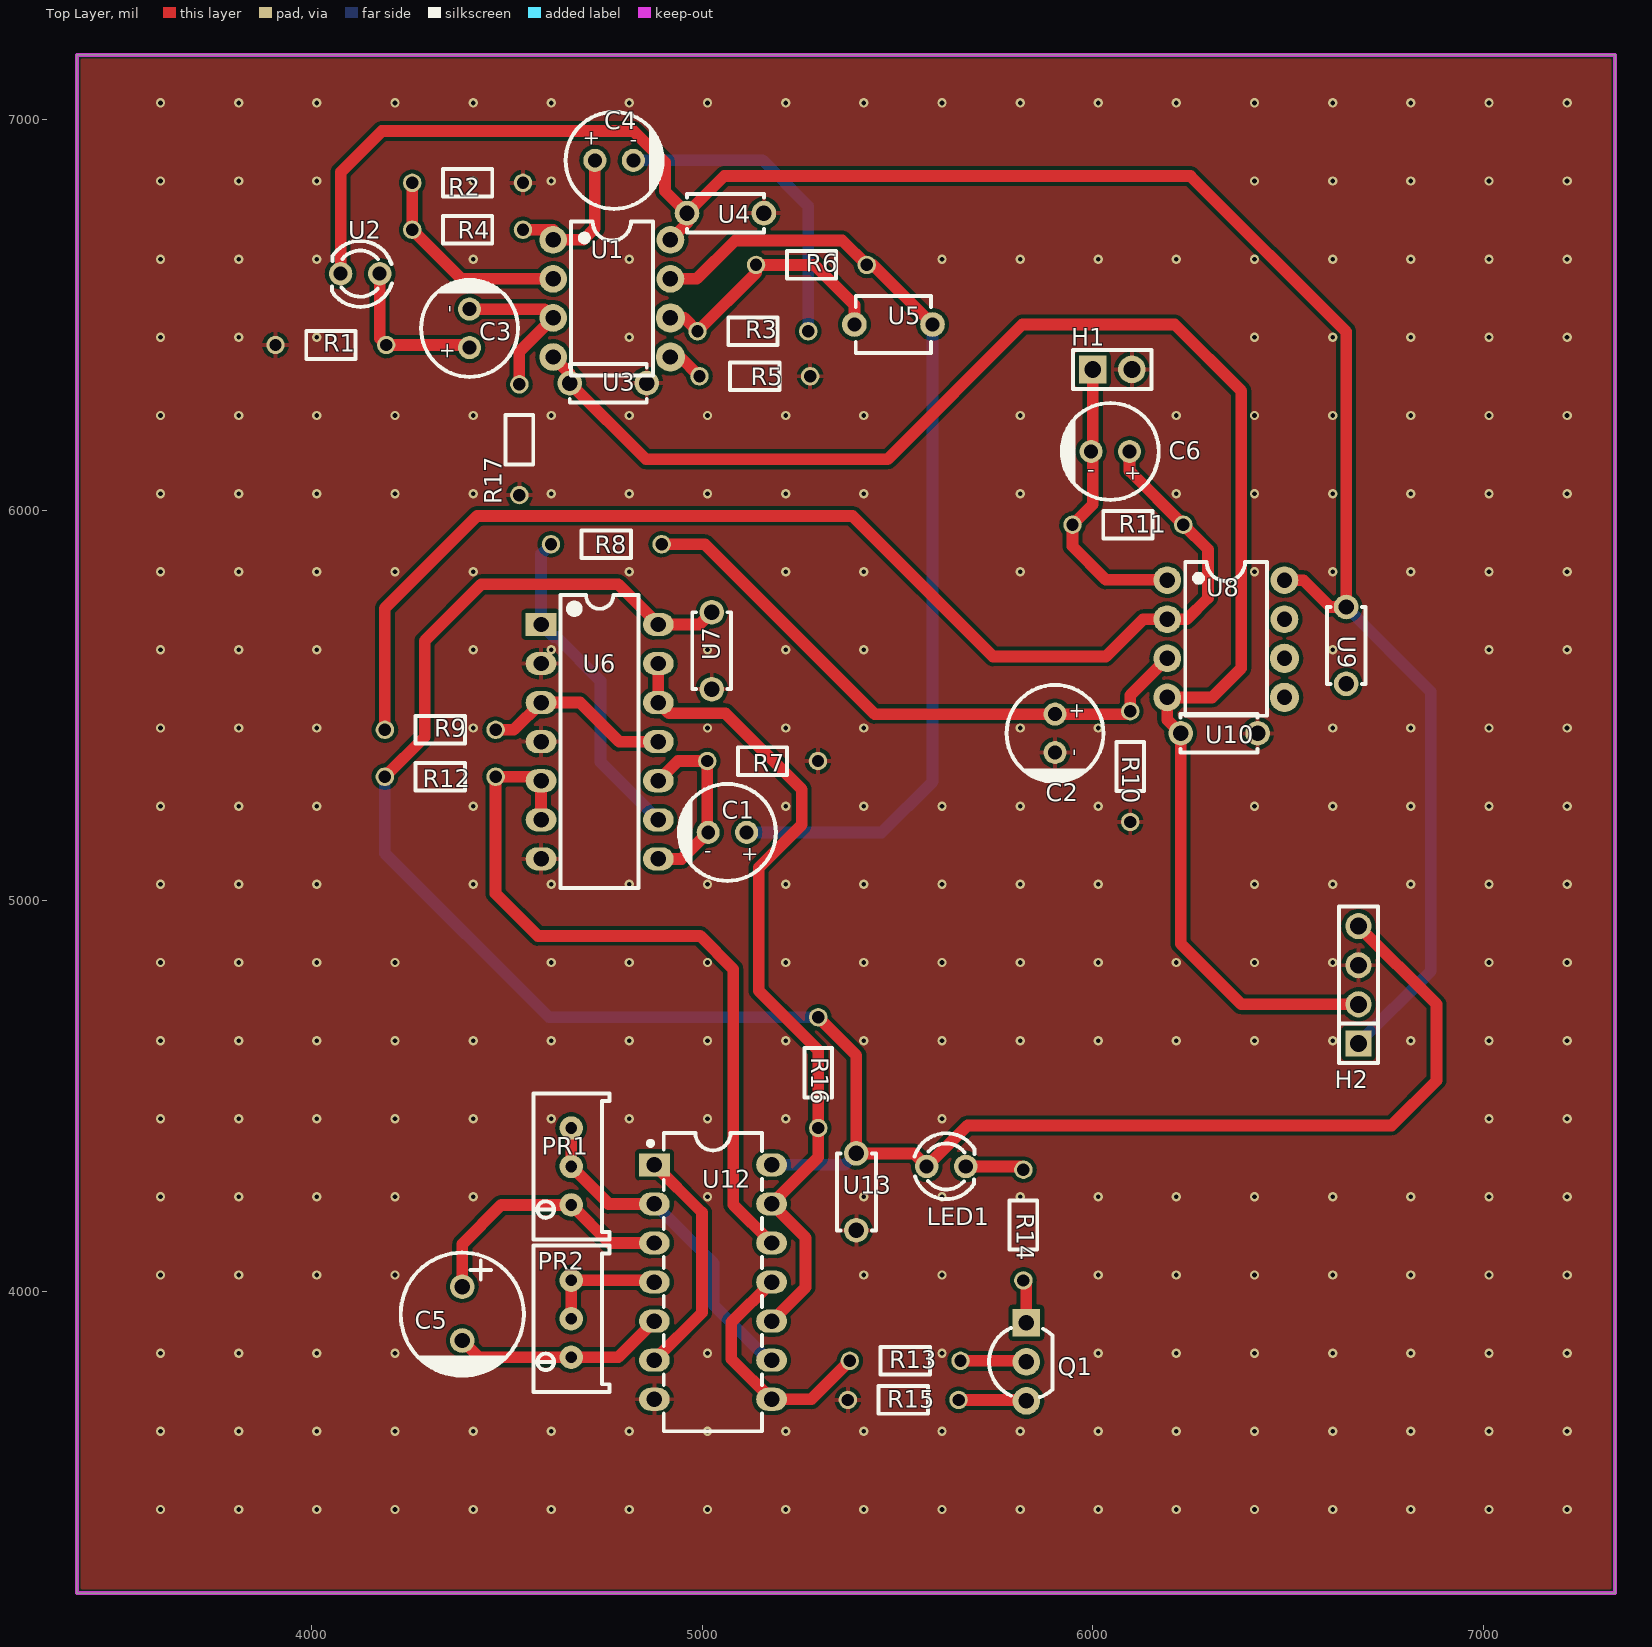
[diagram p0: Top Layer view]
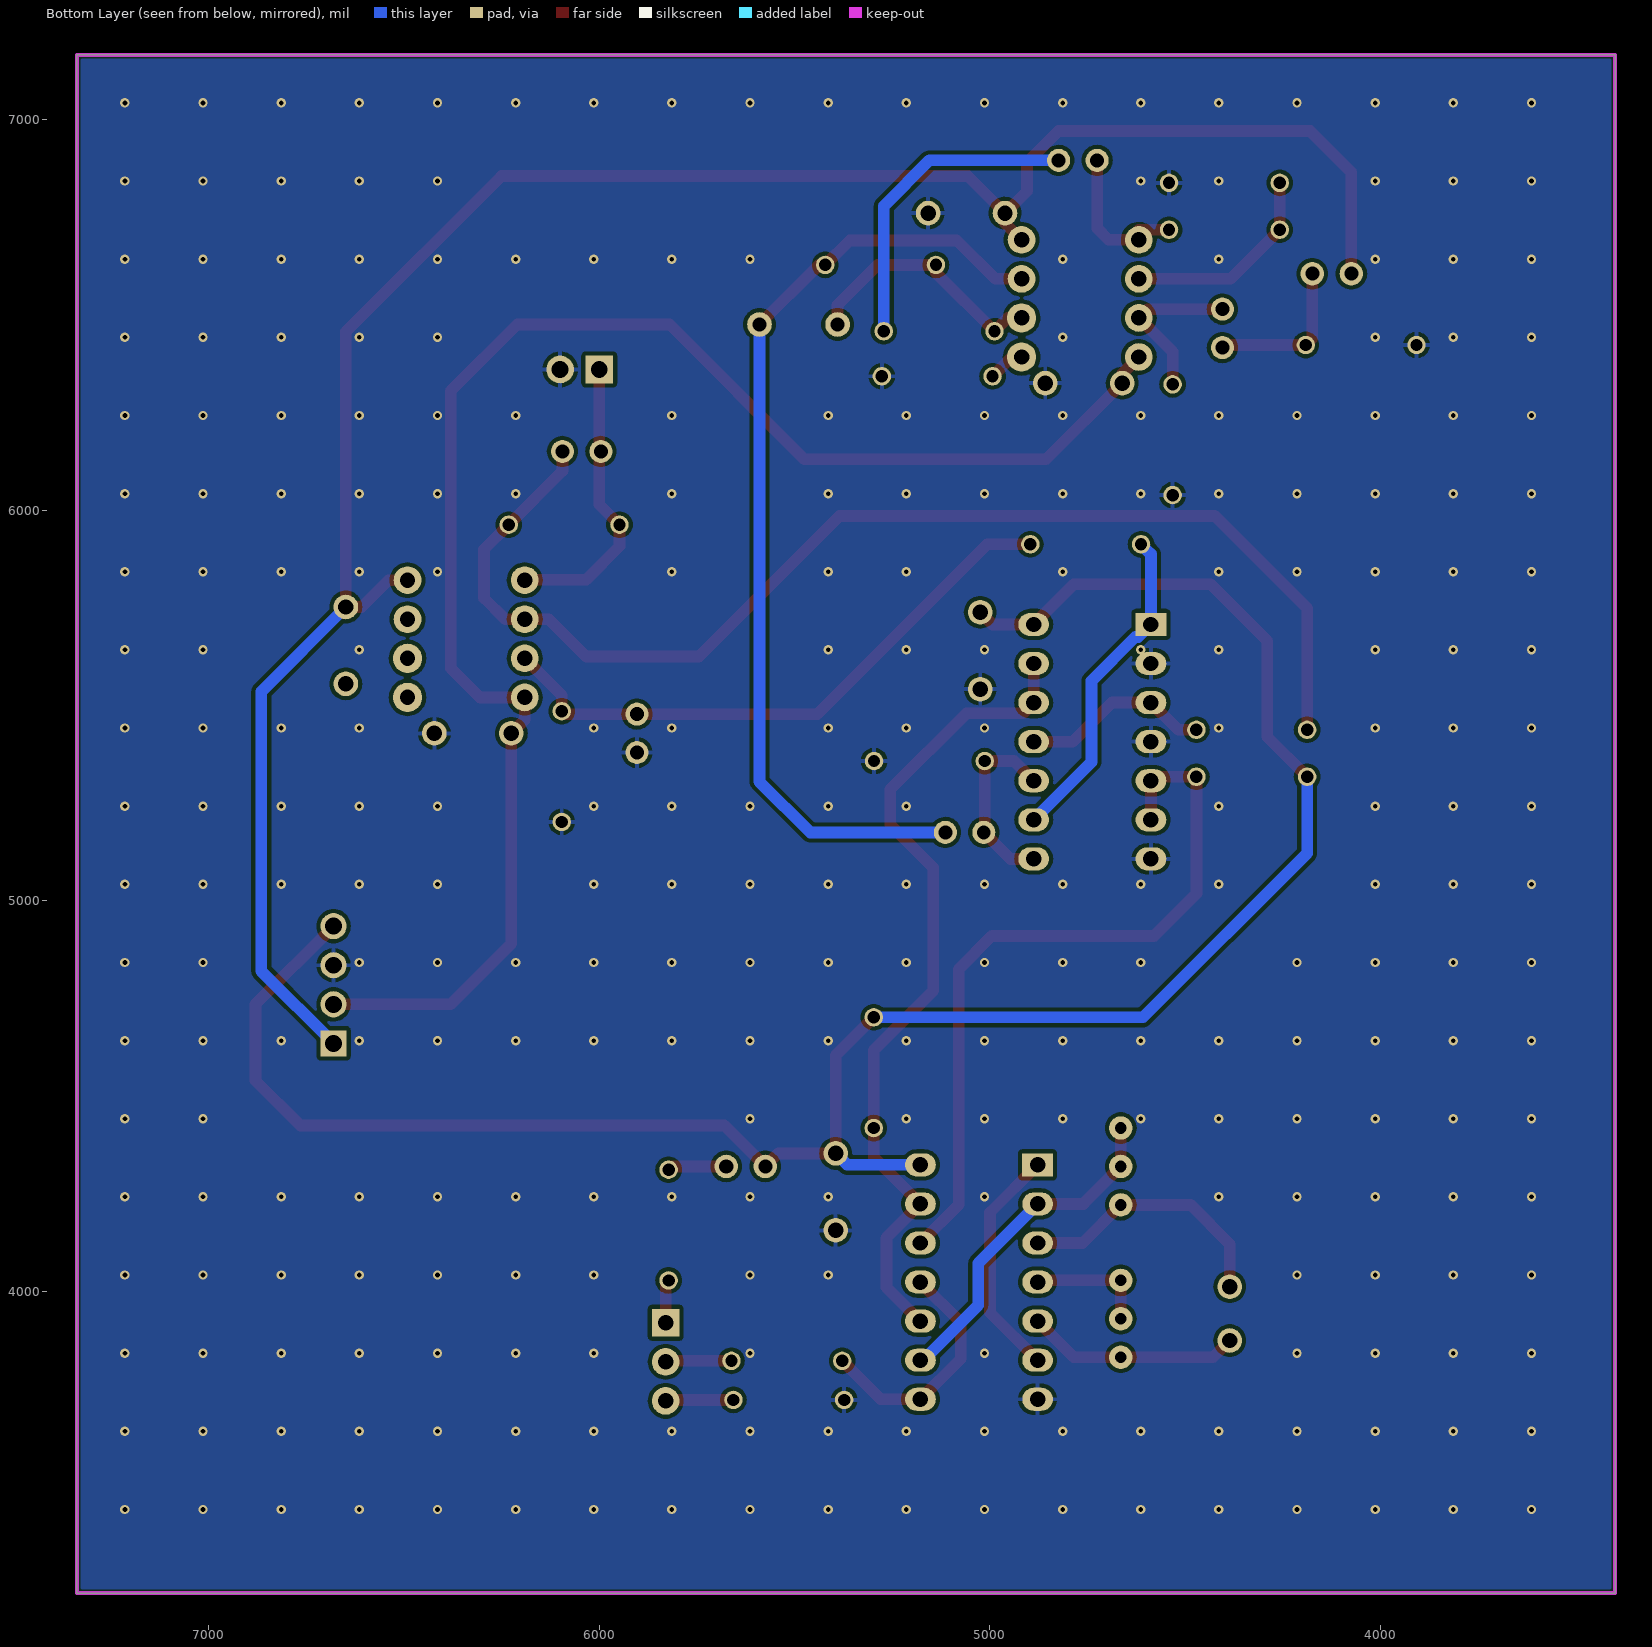
[diagram p1: Bottom Layer view, seen from below]
# Altium PCB MISC51811.pcbdoc
Units mil, origin at the board's own origin, x right, y up, seen from the top; angles counter-clockwise.
Board outline 3937.01 x 3937.01 mil, 2 copper layers (Top Layer, Bottom Layer), stack 62.206 mil thick; 41 components, 31 nets, 123 pads, 283 vias.

## Layer stack, top to bottom
Top Solder Mask Layer: solder mask 0.394, Dk 3.3
Top Layer: signal copper 1.379
Dielectric1: surface 59.449, FR4, Dk 4.5
Bottom Layer: signal copper 1.378
Bottom Solder Mask Layer: solder mask 0.394, Dk 3.3

## Board outline
3400,7165 3400,3227.99 7337.01,3227.99 7337.01,7165

## Design rules (kind name [scope] priority, off if disabled: settings)
BoardOutlineClearance copperThickness2oz_1 [All] p2 off: genericclearance=7.99 ignorepadtopadclearanceinfootprint=FALSE except(0: Arc-SplitContinuation Track-SplitContinuation SMDPad-SplitContinuation THPad-SplitContinuation Via-SplitContinuation Fill-SplitContinuation Region-SplitContinuation Poly-SplitContinuation Text-SplitContinuation Hole-SplitContinuation; 5.98: Arc-CutoutEdge SMDPad-CutoutEdge THPad-CutoutEdge Via-CutoutEdge Fill-CutoutEdge Region-CutoutEdge Text-CutoutEdge; 6.93: Hole-OutlineEdge Hole-CutoutEdge; 10: Poly-OutlineEdge Poly-CutoutEdge; 11.81: Arc-OutlineEdge Track-OutlineEdge SMDPad-OutlineEdge THPad-OutlineEdge Via-OutlineEdge Fill-OutlineEdge Region-OutlineEdge Text-OutlineEdge Track-CutoutEdge)
BoardOutlineClearance copperThickness1oz_1 [All] p4: genericclearance=4.02 ignorepadtopadclearanceinfootprint=FALSE except(0: Arc-SplitContinuation Track-SplitContinuation SMDPad-SplitContinuation THPad-SplitContinuation Via-SplitContinuation Fill-SplitContinuation Region-SplitContinuation Poly-SplitContinuation Text-SplitContinuation Hole-SplitContinuation; 6: SMDPad-CutoutEdge THPad-CutoutEdge Via-CutoutEdge Fill-CutoutEdge Region-CutoutEdge Text-CutoutEdge; 6.93: Hole-OutlineEdge Hole-CutoutEdge; 10: Poly-OutlineEdge Poly-CutoutEdge; 11.8: Arc-OutlineEdge Track-OutlineEdge SMDPad-OutlineEdge THPad-OutlineEdge Via-OutlineEdge Fill-OutlineEdge Region-OutlineEdge Text-OutlineEdge; 11.81: Arc-CutoutEdge Track-CutoutEdge)
Clearance copperThickness2oz [All] p1 off: gap=7.99 ignorepadtopadclearanceinfootprint=FALSE except(5.98: SMDPad-Track SMDPad-SMDPad THPad-Track SMDPad-THPad THPad-THPad Track-Via SMDPad-Via THPad-Via Via-Via Fill-Track Region-Track Fill-SMDPad Region-SMDPad Fill-THPad Region-THPad Fill-Via Region-Via Fill-Fill Fill-Region Region-Region Arc-Track Arc-SMDPad Arc-THPad Arc-Via Fill-Arc Region-Arc Arc-Arc Text-Track SMDPad-Text Text-THPad Text-Via Fill-Text Region-Text Arc-Text Text-Text; 6.93: Hole-Track Hole-SMDPad Hole-THPad Hole-Via Fill-Hole Region-Hole Hole-Arc Hole-Text; 10: Poly-Track Poly-SMDPad Poly-THPad Poly-Via Poly-Fill Poly-Region Poly-Poly Poly-Arc Poly-Text Poly-Hole)
Clearance copperThickness1oz [All] p3: gap=4.02 ignorepadtopadclearanceinfootprint=FALSE except(5.98: SMDPad-Track SMDPad-SMDPad THPad-Track SMDPad-THPad THPad-THPad Track-Via SMDPad-Via THPad-Via Via-Via Fill-Track Region-Track Fill-SMDPad Region-SMDPad Fill-THPad Region-THPad Fill-Via Region-Via Fill-Fill Fill-Region Region-Region; 6: Arc-Track Arc-SMDPad Arc-THPad Arc-Via Fill-Arc Region-Arc Arc-Arc Text-Track SMDPad-Text Text-THPad Text-Via Fill-Text Region-Text Arc-Text Text-Text; 6.93: Hole-Track Hole-SMDPad Hole-THPad Hole-Via Fill-Hole Region-Hole Hole-Arc Hole-Text; 10: Poly-Track Poly-SMDPad Poly-THPad Poly-Via Poly-Fill Poly-Region Poly-Poly Poly-Arc Poly-Text Poly-Hole)
DiffPairsRouting differentialPair [All] p1: maxlimit=6 minlimit=6 mostfreqgap=6 toplayer_minwidth=5 toplayer_prefwidth=10 toplayer_maxwidth=100 toplayer_mingap=6 toplayer_prefgap=6 toplayer_maxgap=6 bottomlayer_minwidth=5 bottomlayer_prefwidth=10 bottomlayer_maxwidth=100 bottomlayer_mingap=6 bottomlayer_prefgap=6 bottomlayer_maxgap=6 maxuncoupledlength=10
HoleToHoleClearance otherClearance [All] p1: gap=11.81 allowstackedmicrovias=TRUE
Length netLength [All] p1: minlimit=0 maxlimit=0
MatchedLengths netLengthTolerance [All] p1: tolerance=1000
PasteMaskExpansion pasteMaskExpansion [All] p1: expansion=0
PlaneConnect innerPlane [All] p1: planeconnectstyle=Relief reliefexpansion=20 reliefentries=4 reliefconductorwidth=10 reliefairgap=10
PolygonConnect copperRegion [(InNet('GND'))] p1: connectstyle=Relief reliefconductorwidth=10 reliefentries=4 polygonreliefangle="90 Angle" airgapwidth=10 via.connectstyle=Relief via.reliefconductorwidth=10 via.reliefentries=4 via.polygonreliefangle="90 Angle" via.airgapwidth=10
RoutingVias viaSize [All] p1: holewidth=12.01 width=24.02 viastyle="Through Hole" minholewidth=11.81 minwidth=19.68 maxholewidth=248.03 maxwidth=393.7
SolderMaskExpansion solderMaskExpansion [IsVia] p1: expansion=-1000 istentingtop=TRUE
SolderMaskExpansion solderMaskExpansion [All] p2: expansion=2 istentingtop=FALSE
Width copperThickness2oz_2 [All] p1 off: maxlimit=100 minlimit=8 preferedwidth=10
Width copperThickness1oz_2 [All] p2: maxlimit=100 minlimit=5 preferedwidth=10

## Components (designator, comment, footprint, x,y, rotation, side; value= is the part's Value field where it differs from the comment)
C1 "1uF" CAP-TH_BD6.3-P2.50-D0.5-FD 5065,5175 r180 top
C2 "1uF" CAP-TH_BD6.3-P2.50-D0.5-FD 5903.54,5428.54 r270 top
C3 "1uF" CAP-TH_BD6.3-P2.50-D0.5-FD 4405,6465 r90 top
C4 "1uF" CAP-TH_BD6.3-P2.50-D0.5-FD 4775,6895 r0 top
C5 "2.2uF" CAP-TH_BD8.0-P3.50-D0.5-FD 4386.37,3943.37 r270 top
C6 "200nF" CAP-TH_BD6.3-P2.50-D0.5-FD 6045,6150 r180 top
H1 "" HDR-TH_2P-P2.54-V-M-1 6050,6360 r0 top
H2 "" HDR-TH_4P-P2.54-V-M 6680,4785 r90 top
LED1 "" LED_TH-3mm 5625,4320 r0 top
PR1 "10kΩ" R_3296 4660,4320 r90 top
PR2 "10kΩ" R_3296 4660,3930 r90 top
Q1 "9013" TO-92-3_L4.8-W3.7-P2.54-R 5830,3820 r90 top
R1 "1kΩ" Res_1/8W 4050,6420 r0 top
R2 "1kΩ" Res_1/8W 4400,6840 r180 top
R3 "1kΩ" Res_1/8W 5130.2,6455.17 r0 top
R4 "10kΩ" Res_1/8W 4400,6715 r0 top
R5 "1kΩ" Res_1/8W 5135,6340 r0 top
R6 "10kΩ" Res_1/8W 5280,6625 r0 top
R7 "1kΩ" Res_1/8W 5155,5360 r180 top
R8 "10kΩ" Res_1/8W 4755,5910 r0 top
R9 "10kΩ" Res_1/8W 4330,5440 r180 top
R10 "100kΩ" Res_1/8W 6093.54,5343.54 r270 top
R11 "100kΩ" Res_1/8W 6090,5965 r180 top
R12 "1kΩ" Res_1/8W 4330,5315 r0 top
R13 "3.3kΩ" Res_1/8W 5520,3820 r0 top
R14 "100" Res_1/8W 5825,4170 r90 top
R15 "50" Res_1/8W 5515,3720 r0 top
R16 "1kΩ" Res_1/8W 5295,4560 r270 top
R17 "1kΩ" Res_1/8W 4535,6180 r90 top
U1 "LF353DRE4" SOIC-8_L5.0-W4.0-P1.27-LS6.1-BL 4769.1,6541.73 r270 top
U2 "DY-PD204-6B" LED-TH_BD3.0-P2.54-FD 4125,6605 r180 top
U3 "100nF" CAP-TH_L5.0-W2.5-P5.00-D1.0 4760,6325 r0 top
U4 "100nF" CAP-TH_L5.0-W2.5-P5.00-D1.0 5060,6760 r0 top
U5 "200pF" CAP-TH_L4.9-W3.7-P5.08-D0.5 5490,6475 r0 top
U6 "MAX4066AESD+" SOIC-14_L8.7-W3.9-P1.27-LS6.0-BL 4738.1,5407.19 r270 top
U7 "100nF" CAP-TH_L5.0-W2.5-P5.00-D1.0 5025,5640 r270 top
U8 "LF353DRE4" SOIC-8_L5.0-W4.0-P1.27-LS6.1-BL 6340.73,5670.5 r270 top
U9 "100nF" CAP-TH_L5.0-W2.5-P5.00-D1.0 6648.54,5653.54 r90 top
U10 "100nF" CAP-TH_L5.0-W2.5-P5.00-D1.0 6323.54,5428.54 r180 top
U12 "SN7404N" PDIP-14_L19.3-W6.4-P2.54-LS7.9-BL-1 5028.02,4024.1 r270 top
U13 "100nF" CAP-TH_L5.0-W2.5-P5.00-D1.0 5395,4255 r90 top

## Footprints (in the part's own frame and the unit in brackets; to place one, negate y for a bottom-side part, rotate by r counter-clockwise, add the part's x,y. Pads: shape width x height; smd on the part's side, far side on the other; paste and mask are expansions set on the pad)
CAP-TH_BD6.3-P2.50-D0.5-FD [mm]
  round 1.5 hole 0.9 paste+0 mask+0.05: 1(-1.25,0) 2(1.25,0)
  silkscreen extent -3.15,-3.15 3.21,3.15
CAP-TH_BD8.0-P3.50-D0.5-FD [mm]
  round 1.6 hole 1: 1(-1.75,0) 2(1.75,0)
  silkscreen extent -3.96,-4 4.04,4
CAP-TH_L4.9-W3.7-P5.08-D0.5 [mm]
  round 1.6 hole 0.9: 1(-2.54,0) 2(2.54,0)
  silkscreen extent -2.45,-1.85 2.45,1.85
CAP-TH_L5.0-W2.5-P5.00-D1.0 [mm]
  round 1.6 hole 1: 1(-2.5,0) 2(2.5,0)
  silkscreen extent -2.5,-1.27 2.5,1.25
HDR-TH_2P-P2.54-V-M-1 [mm]
  rect 1.8x1.8 hole 1.1: 1(-1.27,0)
  round 1.8 hole 1.1: 2(1.27,0)
  silkscreen extent -2.54,-1.27 2.54,1.27
HDR-TH_4P-P2.54-V-M [mm]
  rect 1.7x1.7 hole 1.1: 1(-3.81,0)
  round 1.7 hole 1.1: 2(-1.27,0) 3(1.27,0) 4(3.81,0)
  silkscreen extent -5.08,-1.27 5.08,1.27
LED-TH_BD3.0-P2.54-FD [mil]
  round 60 hole 36 paste+0 mask+1.97: 1(-50,0) 2(50,0)
  silkscreen extent -81,-84 72,85
LED_TH-3mm [mil]
  round 60 hole 36 paste+0 mask+2: 1(-50,0) 2(50,0)
  silkscreen extent -81,-84 72,85
PDIP-14_L19.3-W6.4-P2.54-LS7.9-BL-1 [mm]
  rect 1.5x2 hole 1: 1(-7.62,-3.81)
  oval 1.5x2 hole 1: 2(-5.08,-3.81) 3(-2.54,-3.81) 4(0,-3.81) 5(2.54,-3.81) 6(5.08,-3.81) 7(7.62,-3.81)
  oval 1.5x2 hole 1 copper offset 0,0: 8(7.62,3.81) 9(5.08,3.81) 10(2.54,3.81) 11(0,3.81) 12(-2.54,3.81) 13(-5.08,3.81) 14(-7.62,3.81)
  silkscreen extent -9.7,-4.21 9.7,3.2
R_3296 [mil]
  round 60 hole 30 paste+0 mask+2: 1(-98.4,-5) 2(0,-5) 3(98.4,-5)
  silkscreen extent -187,-103 187,92
Res_1/8W [mil]
  round 47.2 hole 31.5 paste+0 mask+2: 1(-141.7,2.48) 2(141.7,2.48)
  silkscreen extent -63,-33 63,38
SOIC-8_L5.0-W4.0-P1.27-LS6.1-BL [mm]
  round 1.8 hole 1: 1(-3.81,-3.81) 2(-1.27,-3.81) 3(1.27,-3.81) 4(3.81,-3.81) 7(-1.27,3.81) 8(-3.81,3.81)
  round 1.905 hole 1: 5(3.81,3.81) 6(1.27,3.81)
  silkscreen extent -5,-2.64 5,2.67
SOIC-14_L8.7-W3.9-P1.27-LS6.0-BL [mm]
  rect 1.5x2 hole 1: 1(-7.62,-3.81)
  oval 1.5x2 hole 1: 2(-5.08,-3.81) 3(-2.54,-3.81) 4(0,-3.81) 5(2.54,-3.81) 6(5.08,-3.81) 7(7.62,-3.81) 8(7.62,3.81) 9(5.08,3.81) 10(2.54,3.81) 11(0,3.81) 12(-2.54,3.81) 13(-5.08,3.81) 14(-7.62,3.81)
  silkscreen extent -9.53,-2.55 9.53,2.53
TO-92-3_L4.8-W3.7-P2.54-R [mm]
  rect 1.8x1.8 hole 1: 1(2.54,0)
  round 1.8 hole 1: 2(0,0) 3(-2.54,0)
  silkscreen extent -2.3,-1.7 2.2,2.41

## Via types
v1: diameter 24.02, hole 12, Top Layer to Bottom Layer, 283 vias

## Nets (pads, with @x,y where several pads share a name; then routed paths per layer and width w, separated by ;. In a path a pad name is that pad's centre, name@x,y a point inside that pad or via, vN(x,y) a via of type N, cw(c..) or ccw(c..) an arc to the next point about the centre after c; other vN are vias at no path point)
$1N1: R2.2 R4.1 U1.2 | length 532.9
  Top Layer w30: R2.2 R4.1 4384.05,6591.73 U1.2
$1N7: C3.1 R1.2 U2.1 | length 405.5
  Top Layer w30: U2.1 4175,6439.18 R1.2 4398.31,6422.48 C3.1
$1N8: C3.2 R17.2 U1.3 | length 429.3
  Top Layer w30: C3.2 4596.62,6514.21 U1.3 4532.52,6405.15 R17.2
$1N9: C4.1 R4.2 U1.1 | length 370.3
  Top Layer w30: R4.2 U1.1@4619.1,6717.48 ; U1.1 4696.73,6691.73 4725.79,6720.79 C4.1
$1N10: C4.2 R3.2 | length 816.6
  Bottom Layer w30: C4.2 5155,6895 5271.9,6778.1 R3.2
$1N13: R5.1 U1.5 | length 94.6
  Top Layer w30: U1.5 4944.05,6391.73 R5.1
$1N15: R3.1 R6.1 U1.6 U5.1 | length 659.5
  Top Layer w30: U1.6 4954.42,6491.73 R3.1 5138.3,6607.45 R6.1 5287.52,6627.48 5390,6525 U5.1
$1N16: C1.2 R7.2 U6.8 U6.10 | length 485.4
  Top Layer w30: U6.8 4947.98,5107.19 C1.2 5013.3,5177.49 R7.2 4938.43,5357.52 U6.10
$1N17: C1.1 R6.2 U1.7 U5.2 | length 2500.3
  Top Layer w30: U1.7 4986.73,6591.73 5085,6690 5359.18,6690 R6.2 5437.52,6627.48 U5.2
  Bottom Layer w30: C1.1 5460,5175 5590,5305 U5.2
$1N19: R16.2 U6.12 U6.13 U12.10 U12.13 | length 2150.1
  Top Layer w30: U6.13 U6.12 4915.29,5480 5060,5480 5255,5285 5255,5195 5145,5085 5145,4770 5297.48,4617.52 R16.2 5297.48,4343.55 U12.13 5265,4137.12 5265,4011.07 U12.10
$1N21: R8.1 U6.1 U6.9 | length 844.4
  Bottom Layer w30: R8.1 4588.1,5887.27 U6.1 4620.21,5675.08 4627.77,5675.08 4740,5562.85 4740,5355.29 U6.9
$1N22: R12.2 U6.5 U6.6 U12.12 | length 1949.7
  Top Layer w30: U6.6 U6.5 4577.81,5317.48 R12.2 4471.7,5018.3 4580,4910 4995,4910 5080,4825 5080,4222.12 U12.12
$1N23: R9.1 U6.3 U6.11 | length 486.7
  Top Layer w30: R9.1 4518.43,5437.52 U6.3 4687.81,5507.19 4787.81,5407.19 U6.11
$1N26: C2.1 R8.2 R10.1 U8.3 | length 1557
  Top Layer w30: R8.2 5007.52,5912.48 5442.25,5477.75 5903.54,5477.75 6088.52,5477.75 R10.1 6096.01,5525.79 U8.3
$1N27: C6.1 R9.2 R11.1 U8.2 | length 3184.8
  Top Layer w30: R9.2 4188.3,5748.3 4425,5985 5385,5985 5744.89,5625.11 6033.54,5625.11 6128.93,5720.5 U8.2 6240.5,5720.5 6295,5775 6295,5899.22 R11.1 6094.21,6100.01 C6.1
$1N38: PR1.2 PR1.3 U12.2 U12.9 | length 879.6
  Top Layer w30: PR1.3 PR1.2 4760.9,4224.1 U12.2
  Bottom Layer w30: U12.2 5030,4072.12 5030,3965 5170.9,3824.1 U12.9
$1N39: C5.1 PR1.1 U12.3 | length 682.7
  Top Layer w30: C5.1 4386.37,4121.37 4486.6,4221.6 PR1.1 4762.5,4124.1 U12.3
$1N40: PR2.2 PR2.3 U12.4 | length 313.2
  Top Layer w30: PR2.2 PR2.3 4873.72,4028.4 U12.4
$1N41: C5.2 PR2.1 U12.5 | length 547.7
  Top Layer w30: C5.2 4429.24,3831.6 PR2.1 4785.53,3831.6 U12.5
$1N42: U12.1 U12.6 | length 601
  Top Layer w30: U12.6 5000,3946.07 5000,4202.13 U12.1
$1N43: Q1.2 R13.2 | length 169.3
  Top Layer w30: R13.2 5827.52,3822.48 Q1.2
$1N44: Q1.1 R14.1 | length 111.4
  Top Layer w30: R14.1 5830,4020.82 Q1.1
$1N45: LED1.2 R14.2 | length 151
  Top Layer w30: LED1.2 5814.22,4320 R14.2
$1N47: Q1.3 R15.2 | length 174.3
  Top Layer w30: R15.2 5827.52,3722.48 Q1.3
$1N57: R13.1 U12.8 U12.11 | length 626.4
  Top Layer w30: U12.11 5075,3921.07 5075,3827.12 U12.8 5279.92,3724.1 R13.1
+5V: H2.4 LED1.1 R12.1 R16.1 U6.14 U7.1 U12.14 U13.2 | length 5404.8
  Top Layer w30: R12.1 4290,5419.18 4290,5665 4435,5810 4785.29,5810 U6.14 4993.77,5707.19 U7.1 ; R16.1 5395,4604.18 U13.2 5541.57,4353.43 LED1.1 5680,4425 6765,4425 6880,4540 6880,4735 H2.4
  Bottom Layer w30: R12.1 4188.3,5121.7 4608.3,4701.7 R16.1 ; U12.14 5365.67,4324.1 U13.2
+12V: H2.1 U1.8 U2.2 U4.1 U8.8 U9.2 | length 5471.3
  Top Layer w30: U2.2 4075,6865 4180,6970 4825,6970 4905,6890 4905,6816.57 U4.1 ; U1.8 4961.57,6734.21 U4.1 ; U8.8 6539.5,5820.5 6608.04,5751.96 U9.2 6648.54,6456.46 6250,6855 5056.57,6855 U4.1
  Bottom Layer w30: U9.2 6865,5535.5 6865,4820 H2.1
-12V: H2.2 U1.4 U3.1 U8.4 U10.2 | length 4190.9
  Top Layer w30: U1.4 4661.57,6349.26 U3.1 4856.57,6130 5475,6130 5820,6475 6210,6475 6380,6305 6380,5595 6305.5,5520.5 U8.4 6190.73,5462.92 U10.2 6225.11,4889.89 6380,4735 H2.2
AGND: U9.1
GND: C2.2 H1.2 H2.3 R1.1 R2.1 R5.2 R7.1 R10.2 R15.1 R17.1 U3.2 U4.2 U6.2 U6.4 U6.7 U7.2 U10.1 U12.7 U13.1
  other v1: 3614.1,3442.09 3814.1,3442.09 4014.1,3442.09 4214.1,3442.09 4414.1,3442.09 4614.1,3442.09 4814.1,3442.09 5014.1,3442.09 5214.1,3442.09 5414.1,3442.09 5614.1,3442.09 5814.1,3442.09 6014.1,3442.09 6214.1,3442.09 6414.1,3442.09 6614.1,3442.09 6814.1,3442.09 7014.1,3442.09 7214.1,3442.09 3614.1,3642.09 3814.1,3642.09 4014.1,3642.09 4214.1,3642.09 4414.1,3642.09 4614.1,3642.09 4814.1,3642.09 5014.1,3642.09 5214.1,3642.09 5414.1,3642.09 5614.1,3642.09 5814.1,3642.09 6014.1,3642.09 6214.1,3642.09 6414.1,3642.09 6614.1,3642.09 6814.1,3642.09 7014.1,3642.09 7214.1,3642.09 3614.1,3842.09 3814.1,3842.09 4014.1,3842.09 4214.1,3842.09 5014.1,3842.09 5614.1,3842.09 6014.1,3842.09 6214.1,3842.09 6414.1,3842.09 6614.1,3842.09 6814.1,3842.09 7014.1,3842.09 7214.1,3842.09 3614.1,4042.09 3814.1,4042.09 4014.1,4042.09 4214.1,4042.09 5414.1,4042.09 5614.1,4042.09 6014.1,4042.09 6214.1,4042.09 6414.1,4042.09 6614.1,4042.09 6814.1,4042.09 7014.1,4042.09 7214.1,4042.09 3614.1,4242.09 3814.1,4242.09 4014.1,4242.09 4214.1,4242.09 4414.1,4242.09 5014.1,4242.09 5414.1,4242.09 5614.1,4242.09 5814.1,4242.09 6014.1,4242.09 6214.1,4242.09 6414.1,4242.09 6614.1,4242.09 6814.1,4242.09 7014.1,4242.09 7214.1,4242.09 3614.1,4442.09 3814.1,4442.09 4014.1,4442.09 4214.1,4442.09 4414.1,4442.09 4614.1,4442.09 4814.1,4442.09 5014.1,4442.09 5214.1,4442.09 5614.1,4442.09 7014.1,4442.09 7214.1,4442.09 3614.1,4642.09 3814.1,4642.09 4014.1,4642.09 4214.1,4642.09 4414.1,4642.09 4614.1,4642.09 4814.1,4642.09 5014.1,4642.09 5214.1,4642.09 5414.1,4642.09 5614.1,4642.09 5814.1,4642.09 6014.1,4642.09 6214.1,4642.09 6414.1,4642.09 6614.1,4642.09 6814.1,4642.09 7014.1,4642.09 7214.1,4642.09 3614.1,4842.09 3814.1,4842.09 4014.1,4842.09 4214.1,4842.09 4614.1,4842.09 4814.1,4842.09 5014.1,4842.09 5214.1,4842.09 5414.1,4842.09 5614.1,4842.09 5814.1,4842.09 6014.1,4842.09 6214.1,4842.09 6414.1,4842.09 6614.1,4842.09 7014.1,4842.09 7214.1,4842.09 3614.1,5042.09 3814.1,5042.09 4014.1,5042.09 4414.1,5042.09 4614.1,5042.09 4814.1,5042.09 5014.1,5042.09 5214.1,5042.09 5414.1,5042.09 5614.1,5042.09 5814.1,5042.09 6014.1,5042.09 6414.1,5042.09 6614.1,5042.09 6814.1,5042.09 7014.1,5042.09 7214.1,5042.09 3614.1,5242.09 3814.1,5242.09 4014.1,5242.09 4414.1,5242.09 5214.1,5242.09 5414.1,5242.09 5614.1,5242.09 5814.1,5242.09 6014.1,5242.09 6414.1,5242.09 6614.1,5242.09 6814.1,5242.09 7014.1,5242.09 7214.1,5242.09 3614.1,5442.09 3814.1,5442.09 4014.1,5442.09 4414.1,5442.09 5014.1,5442.09 5214.1,5442.09 5414.1,5442.09 5814.1,5442.09 6014.1,5442.09 6614.1,5442.09 6814.1,5442.09 7014.1,5442.09 7214.1,5442.09 3614.1,5642.09 3814.1,5642.09 4014.1,5642.09 4414.1,5642.09 4614.1,5642.09 5014.1,5642.09 5214.1,5642.09 5414.1,5642.09 6614.1,5642.09 7014.1,5642.09 7214.1,5642.09 3614.1,5842.09 3814.1,5842.09 4014.1,5842.09 4214.1,5842.09 4414.1,5842.09 4814.1,5842.09 5214.1,5842.09 5414.1,5842.09 5814.1,5842.09 6414.1,5842.09 6614.1,5842.09 6814.1,5842.09 7014.1,5842.09 7214.1,5842.09 3614.1,6042.09 3814.1,6042.09 4014.1,6042.09 4214.1,6042.09 4414.1,6042.09 4614.1,6042.09 4814.1,6042.09 5014.1,6042.09 5214.1,6042.09 5414.1,6042.09 5814.1,6042.09 6214.1,6042.09 6414.1,6042.09 6614.1,6042.09 6814.1,6042.09 7014.1,6042.09 7214.1,6042.09 3614.1,6242.09 3814.1,6242.09 4014.1,6242.09 4214.1,6242.09 4414.1,6242.09 4614.1,6242.09 4814.1,6242.09 5014.1,6242.09 5214.1,6242.09 5414.1,6242.09 5814.1,6242.09 6214.1,6242.09 6414.1,6242.09 6614.1,6242.09 6814.1,6242.09 7014.1,6242.09 7214.1,6242.09 3614.1,6442.09 3814.1,6442.09 4014.1,6442.09 4814.1,6442.09 6414.1,6442.09 6614.1,6442.09 6814.1,6442.09 7014.1,6442.09 7214.1,6442.09 3614.1,6642.09 3814.1,6642.09 4014.1,6642.09 4414.1,6642.09 4814.1,6642.09 5614.1,6642.09 5814.1,6642.09 6014.1,6642.09 6214.1,6642.09 6414.1,6642.09 6614.1,6642.09 6814.1,6642.09 7014.1,6642.09 7214.1,6642.09 3614.1,6842.09 3814.1,6842.09 4014.1,6842.09 4414.1,6842.09 4614.1,6842.09 6414.1,6842.09 6614.1,6842.09 6814.1,6842.09 7014.1,6842.09 7214.1,6842.09 3614.1,7042.09 3814.1,7042.09 4014.1,7042.09 4214.1,7042.09 4414.1,7042.09 4614.1,7042.09 4814.1,7042.09 5014.1,7042.09 5214.1,7042.09 5414.1,7042.09 5614.1,7042.09 5814.1,7042.09 6014.1,7042.09 6214.1,7042.09 6414.1,7042.09 6614.1,7042.09 6814.1,7042.09 7014.1,7042.09 7214.1,7042.09
OUT: C6.2 H1.1 R11.2 U8.1 | length 752.1
  Top Layer w30: H1.1 6000,6014.22 R11.2 5948.3,5907.2 6033.54,5821.96 6187.57,5821.96 U8.1@6189.88,5819.65
pads on no net: U8.5 U8.6 U8.7

## Polygon pours and split planes (outlines as drawn)
GND on Top Layer (solid, remove dead copper, pour order 0): 3000,7475 3000,3000 7740,3000 7740,7475
GND on Bottom Layer (solid, remove dead copper, pour order 2): 3185,7380 3185,3105 7505,3105 7505,7380

## Keep-outs
Board Outline Layer:
  the board outline again, w10